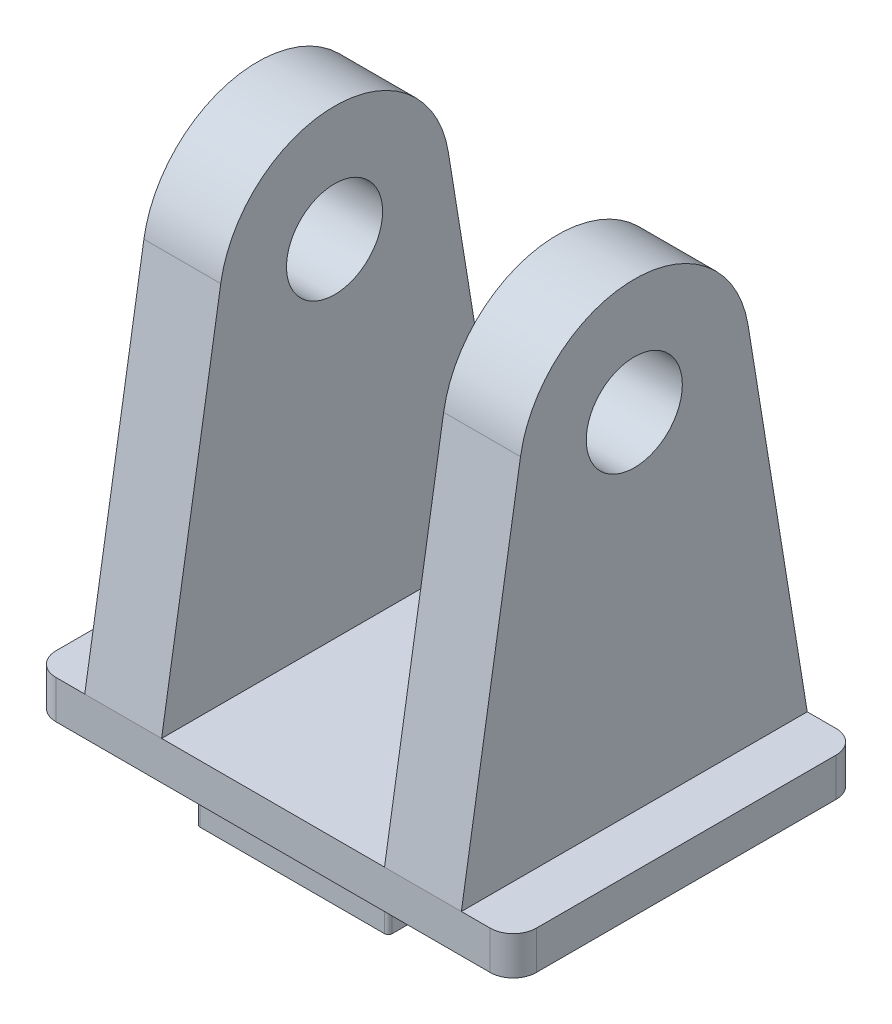
from build123d import *

# Parameters (mm, degrees)
BOSS_EXTRUDE_1_DEPTH = 20
BOSS_EXTRUDE_2_DEPTH = 20
BOSS_EXTRUDE_START   = 58
SKETCH_3_R           = 25
BOSS_EXTRUDE_3_DEPTH = 40


with BuildPart() as part:
    # Sketch 1 → Boss-Extrude 1 (new body)
    with BuildSketch(Plane(origin=(0, 0, 0), x_dir=(1, 0, 0), z_dir=(0, 1, 0))):
        with BuildLine():
            Line((113, 90), (-113, 90))
            ThreePointArc((-113, 90), (-121.485281374, 86.485281374), (-125, 78))
            Line((-125, 78), (-125, -78))
            ThreePointArc((-125, -78), (-121.485281374, -86.485281374), (-113, -90))
            Line((-113, -90), (113, -90))
            ThreePointArc((113, -90), (121.485281374, -86.485281374), (125, -78))
            Line((125, -78), (125, 78))
            ThreePointArc((125, 78), (121.485281374, 86.485281374), (113, 90))
        make_face()
    extrude(amount=BOSS_EXTRUDE_1_DEPTH)

    # Sketch 2 → Boss-Extrude 2 (add)
    with BuildSketch(Plane.XZ):
        with BuildLine():
            Line((48, 80), (-48, 80))
            ThreePointArc((-48, 80), (-49.414213562, 79.414213562), (-50, 78))
            Line((-50, 78), (-50, -78))
            ThreePointArc((-50, -78), (-49.414213562, -79.414213562), (-48, -80))
            Line((-48, -80), (48, -80))
            ThreePointArc((48, -80), (49.414213562, -79.414213562), (50, -78))
            Line((50, -78), (50, 78))
            ThreePointArc((50, 78), (49.414213562, 79.414213562), (48, 80))
        make_face()
    extrude(amount=BOSS_EXTRUDE_2_DEPTH)

    # Sketch 3 → Boss-Extrude 3 (add)
    with BuildSketch(Plane(origin=(0, 0, 0), x_dir=(0, 0, -1), z_dir=(1, 0, 0)).offset(BOSS_EXTRUDE_START)):
        with BuildLine():
            Line((-59.224993899, 209.61249695), (-90, 20))
            Line((-90, 20), (90, 20))
            Line((90, 20), (59.224993899, 209.61249695))
            ThreePointArc((59.224993899, 209.61249695), (0, 260), (-59.224993899, 209.61249695))
        make_face()
        with Locations((0, 200)):
            Circle(SKETCH_3_R, mode=Mode.SUBTRACT)
    boss_extrude_3 = extrude(amount=BOSS_EXTRUDE_3_DEPTH)

    # Mirror 1: Boss-Extrude 3 across plane
    add(boss_extrude_3.mirror(Plane(origin=(0, 0, 0), x_dir=(0, 0, 1), z_dir=(1, 0, 0))))


solid = part.part
